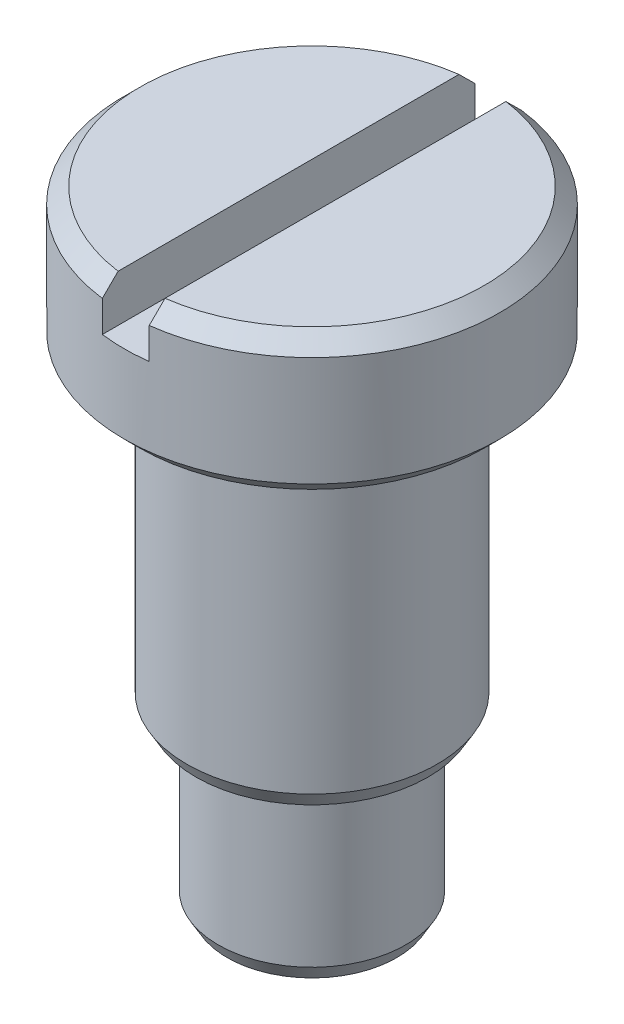
from build123d import *
from OCP.BRepFilletAPI import BRepFilletAPI_MakeChamfer

# Parameters (mm, degrees)
CHAMFER1_SIZE      = 1
CHAMFER2_SIZE      = 1
CHAMFER2_SIZE2     = 0.577350269
SKETCH2_W          = 3
SKETCH2_H          = 30.588331256
CUT_EXTRUDE1_DEPTH = 3


with BuildPart() as part:
    # Sketch1 → Revolve1 (revolve)
    with BuildSketch(Plane.XY, mode=Mode.PRIVATE) as revolve1_sk:
        Polygon((0, 0), (0, 40), (12, 40), (12, 31), (8, 31), (8, 11), (6, 11), (6, 0), align=None)
    revolve(revolve1_sk.sketch.rotate(Axis((0, 0, 0), (0, 1, 0)), 90), axis=Axis((0, 0, 0), (0, 1, 0)))

    # Chamfer1
    chamfer1_edges = [part.edges().sort_by_distance(p)[0] for p in [
        (0, 31, 12),
        (0, 40, 12),
    ]]
    chamfer(chamfer1_edges, length=CHAMFER1_SIZE)

    # Chamfer2: one chamfer whose edges measure the first distance from different faces: ONE call of the kernel's chamfer builder (chamfer() names one face for all edges)
    chamfer2_edges_1 = [part.edges().sort_by_distance(p)[0] for p in [
        (0, 0, 6),
    ]]
    chamfer2_side_1 = [part.faces().sort_by_distance(p)[0] for p in [
        (0, 5.5, 6),
    ]]
    chamfer2_edges_2 = [part.edges().sort_by_distance(p)[0] for p in [
        (0, 11, 8),
    ]]
    chamfer2_side_2 = [part.faces().sort_by_distance(p)[0] for p in [
        (0, 21, 8),
    ]]
    chamfer2 = BRepFilletAPI_MakeChamfer(part.part.solid().wrapped)
    for e in chamfer2_edges_1:
        chamfer2.Add(CHAMFER2_SIZE, CHAMFER2_SIZE2, e.wrapped, chamfer2_side_1[0].wrapped)  # the first distance lies on this face
    for e in chamfer2_edges_2:
        chamfer2.Add(CHAMFER2_SIZE, CHAMFER2_SIZE2, e.wrapped, chamfer2_side_2[0].wrapped)  # the first distance lies on this face
    add(Compound.cast(chamfer2.Shape()), mode=Mode.REPLACE)

    # Sketch2 → Cut-Extrude1 (cut)
    with BuildSketch(Plane(origin=(0, 40, 0), x_dir=(1, 0, 0), z_dir=(0, 1, 0))):
        Rectangle(SKETCH2_W, SKETCH2_H)
    extrude(amount=-CUT_EXTRUDE1_DEPTH, mode=Mode.SUBTRACT)


solid = part.part
